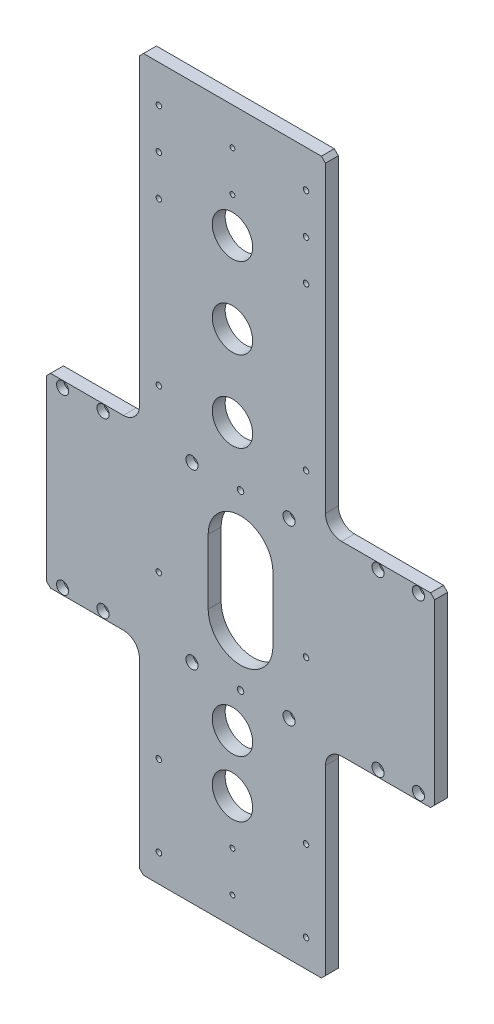
SolidWorks part; units mm, degrees
material "6061 合金"
ref_plane "Front" through (0, 0, 0) normal (0, 0, 1) x (1, 0, 0)
ref_plane "Top" through (0, 0, 0) normal (0, 1, 0) x (1, 0, 0)
ref_plane "Right" through (0, 0, 0) normal (1, 0, 0) x (0, 0, -1)
sketch "草图1" plane through (0, 0, 0) normal (0, 0, 1) x (1, 0, 0)
  line L1 (-240, -115) -> (240, -115)
  line L2 (-240, -115) -> (-240, 115)
  line L3 (-240, 115) -> (240, 115)
  line L4 (240, -115) -> (240, 115)
  line L5 (-240, -115) -> (240, 115) construction
  line L6 (-240, 115) -> (240, -115) construction
  line L7 (-125, 515) -> (105, 515)
  line L8 (-125, 515) -> (-125, 115)
  line L9 (-125, 115) -> (105, 115)
  line L10 (105, 515) -> (105, 115)
  line L11 (-125, 515) -> (105, 115) construction
  line L12 (-125, 115) -> (105, 515) construction
  line L13 (-125, -365) -> (105, -365)
  line L14 (-125, -365) -> (-125, -115)
  line L15 (-125, -115) -> (105, -115)
  line L16 (105, -365) -> (105, -115)
  line L17 (-125, -365) -> (105, -115) construction
  line L18 (-125, -115) -> (105, -365) construction
  point P0 (0, 0)
  dimension "D1" = 230
  dimension "D2" = 480
  dimension "D3" = 230
  dimension "D4" = 400
  dimension "D5" = 250
  dimension "D6" = 115
extrude "凸台-拉伸1" add sketch "草图1" along normal blind 16 contours L10 L7 L8 L3 | L1 L4 L3 L2 | L13 L16 L1 L14
fillet "圆角1" radius 20 4 edges at (105, 115, 8) (105, -115, 8) (-125, -115, 8) (-125, 115, 8)
hole_wizard "打孔尺寸(%根据)内六角圆柱头螺钉的类型1" positions "草图2" profile "草图3" counterbore size "M8" standard "GB" end condition through all
sketch "草图2" plane through (0, 0, 16) normal (0, 0, 1) x (1, 0, 0)
  line L10 (-240, 0) -> (240, 0) construction
  line L11 (-240, -115) -> (-240, 115) construction
  line L12 (240, -115) -> (240, 115) construction
  line L14 (-220, -107) -> (220, -107) construction
  line L15 (-220, -107) -> (-220, 107) construction
  line L16 (-220, 107) -> (220, 107) construction
  line L17 (220, -107) -> (220, 107) construction
  line L18 (0, 107) -> (0, -107) construction
  line L19 (-220, 0) -> (220, 0) construction
  line L20 (-170, 107) -> (-170, -107) construction
  line L21 (170, 107) -> (170, -107) construction
  line L22 (-60, 107) -> (-60, -107) construction
  line L23 (60, 107) -> (60, -107) construction
  point P318 (220, 107)
  point P505 (-220, -107)
  point P506 (-220, 107)
  point P507 (220, -107)
  point P529 (-170, 107)
  point P530 (-170, -107)
  point P531 (170, 107)
  point P532 (170, -107)
  point P533 (-60, 107)
  point P534 (-60, -107)
  point P535 (60, 107)
  point P536 (60, -107)
  dimension "D1" = 214
  dimension "D2" = 440
  dimension "D3" = 340
  dimension "D4" = 120
  dimension "D5" = 0
sketch "草图3" plane through (60, -107, 16) normal (1, 0, 0) x (0, -1, 0)
  line L0 (0, 0) -> (0, 16)
  line L1 (0, 16) -> (4.5, 16)
  line L3 (4.5, 16) -> (4.5, 9)
  line L4 (4.5, 9) -> (7.5, 9)
  line L5 (7.5, 9) -> (7.5, 0)
  line L7 (7.5, 0) -> (0, 0)
  line L11 (0, -6.35) -> (0, 107.95) construction
  dimension "通孔孔直径" = 9
  dimension "通孔孔深度" = 16
  dimension "柱形沉头孔直径" = 15
  dimension "柱形沉头孔深度" = 9
hole_wizard "大小mm 暗销孔1" positions "草图4" profile "草图5" hole size "Ø8.0" standard "GB" end condition through all
sketch "草图4" plane through (0, 0, 16) normal (0, 0, 1) x (1, 0, 0)
  line L1 (-220, -107) -> (220, -107) construction
  line L2 (-220, -107) -> (-220, 107) construction
  line L3 (-220, 107) -> (220, 107) construction
  line L4 (220, -107) -> (220, 107) construction
  line L5 (0, 107) -> (0, -107) construction
  line L6 (-220, 0) -> (220, 0) construction
  line L7 (-240, 0) -> (240, 0) construction
  line L8 (-240, -115) -> (-240, 115) construction
  line L9 (240, -115) -> (240, 115) construction
  circle A0 centre (220, 107) radius 4.5 construction
  circle A1 centre (-220, 107) radius 4.5 construction
  point P769 (0, -107)
  point P771 (0, 107)
sketch "草图5" plane through (0, 107, 16) normal (1, 0, 0) x (0, -1, 0)
  line L0 (0, 0) -> (0, 16)
  line L1 (0, 16) -> (4, 16)
  line L2 (4, 16) -> (4, 0)
  line L5 (4, 0) -> (0, 0)
  line L11 (0, -6.35) -> (0, 107.95) construction
  dimension "通孔孔直径" = 8
  dimension "通孔孔深度" = 16
hole_wizard "M8 螺纹孔1" positions "草图6" profile "草图7" tap size "M8" standard "GB"
sketch "草图6" plane through (0, 0, 16) normal (0, 0, 1) x (1, 0, 0)
  line L1 (-101, -469) -> (81, -469) construction
  line L2 (-101, -469) -> (-101, 469) construction
  line L3 (-101, 469) -> (81, 469) construction
  line L4 (81, -469) -> (81, 469) construction
  line L5 (-10, 469) -> (-10, -469) construction
  line L6 (-101, 0) -> (81, 0) construction
  line L7 (-10, 515) -> (-10, -365) construction
  line L8 (-125, 515) -> (105, 515) construction
  line L9 (-125, -365) -> (105, -365) construction
  line L10 (-240, 0) -> (240, 0) construction
  line L11 (-240, -115) -> (-240, 115) construction
  line L12 (240, -115) -> (240, 115) construction
  line L13 (81, -469) -> (81, 469) construction
  point P2 (81, 469)
  point P562 (-101, 469)
  point P586 (-101, 169)
  point P588 (-101, 369)
  point P590 (-101, 419)
  point P595 (-101, -31)
  point P597 (-101, -231)
  point P599 (-101, -331)
  point P606 (81, -331)
  point P607 (81, -231)
  point P608 (81, -31)
  point P609 (81, 419)
  point P610 (81, 369)
  point P611 (81, 169)
  dimension "D1" = 182
  dimension "D2" = 200
  dimension "D3" = 46
  dimension "D4" = 50
  dimension "D5" = 50
  dimension "D6" = 200
  dimension "D7" = 200
  dimension "D8" = 100
sketch "草图7" plane through (81, 469, 16) normal (1, 0, 0) x (0, -1, 0)
  line L0 (0, 0) -> (0, 24.2929)
  line L1 (0, 24.2929) -> (3.4, 22.25)
  line L2 (3.4, 22.25) -> (3.4, 0)
  line L5 (3.4, 0) -> (0, 0)
  line L10 (0, 24.2929) -> (-3.4, 22.25) construction
  line L11 (0, -6.35) -> (0, 107.95) construction
  dimension "螺纹孔钻头直径" = 6.8
  dimension "螺纹孔钻头深度" = 22.25
  dimension "导头角度" = 118
cosmetic thread "孔螺蚊线2" parameters "D1"=16, "D2"=8
cosmetic thread "孔螺蚊线3" parameters "D1"=16, "D2"=8
cosmetic thread "孔螺蚊线4" parameters "D1"=16, "D2"=8
cosmetic thread "孔螺蚊线5" parameters "D1"=16, "D2"=8
cosmetic thread "孔螺蚊线6" parameters "D1"=16, "D2"=8
cosmetic thread "孔螺蚊线7" parameters "D1"=16, "D2"=8
cosmetic thread "孔螺蚊线8" parameters "D1"=16, "D2"=8
cosmetic thread "孔螺蚊线9" parameters "D1"=16, "D2"=8
cosmetic thread "孔螺蚊线10" parameters "D1"=16, "D2"=8
cosmetic thread "孔螺蚊线11" parameters "D1"=16, "D2"=8
cosmetic thread "孔螺蚊线12" parameters "D1"=16, "D2"=8
cosmetic thread "孔螺蚊线14" parameters "D1"=16, "D2"=8
cosmetic thread "孔螺蚊线15" parameters "D1"=16, "D2"=8
cosmetic thread "孔螺蚊线16" parameters "D1"=16, "D2"=8
chamfer "倒角1" distance 5 angle 45 8 edges at (240, 115, 8) (240, -115, 8) (105, -365, 8) (-125, -365, 8) (-240, -115, 8) (-240, 115, 8) (-125, 515, 8) (105, 515, 8)
sketch "草图8" plane through (0, 0, 16) normal (0, 0, 1) x (1, 0, 0)
  line L0 (-10, 515) -> (-10, -365) construction
  line L1 (-120, 515) -> (100, 515) construction
  line L2 (-120, -365) -> (100, -365) construction
  line L3 (0, -40) -> (0, 40) construction
  line L6 (-40, -40) -> (-40, 40)
  line L7 (40, -40) -> (40, 40)
  circle A0 centre (-10, 375) radius 25
  circle A2 centre (-10, -155) radius 25
  circle A3 centre (-10, -225) radius 25
  circle A4 centre (-10, 275) radius 25
  circle A8 centre (-10, 175) radius 25
  arc A9 (-40, -40) -> (40, -40) centre (0, -40) ccw
  arc A10 (40, 40) -> (-40, 40) centre (0, 40) ccw
  point P18 (0, 0)
  dimension "D1" = 50
  dimension "D2" = 100
  dimension "D3" = 70
  dimension "D5" = 100
  dimension "D6" = 140
  dimension "D4" = 140
  dimension "D7" = 80
  dimension "D8" = 80
extrude "切除-拉伸1" cut sketch "草图8" against normal through all
hole_wizard "大小mm 暗销孔4" positions "草图9" profile "草图10" hole size "Ø6.0" standard "GB" end condition through all
sketch "草图9" plane through (0, 0, 16) normal (0, 0, 1) x (1, 0, 0)
  line L0 (-101, -331) -> (81, -331) construction
  line L1 (-10, -331) -> (-10, -281) construction
  line L2 (-101, 469) -> (81, 469) construction
  line L3 (-101, 419) -> (81, 419) construction
  point P6 (-10, -331)
  point P11 (-10, -281)
  point P22 (-10, 469)
  point P31 (-10, 419)
  dimension "D1" = 50
sketch "草图10" plane through (-10, 419, 16) normal (1, 0, 0) x (0, -1, 0)
  line L0 (0, 0) -> (0, 16)
  line L1 (0, 16) -> (3, 16)
  line L2 (3, 16) -> (3, 0)
  line L5 (3, 0) -> (0, 0)
  line L11 (0, -6.35) -> (0, 107.95) construction
  dimension "通孔孔直径" = 6
  dimension "通孔孔深度" = 16
